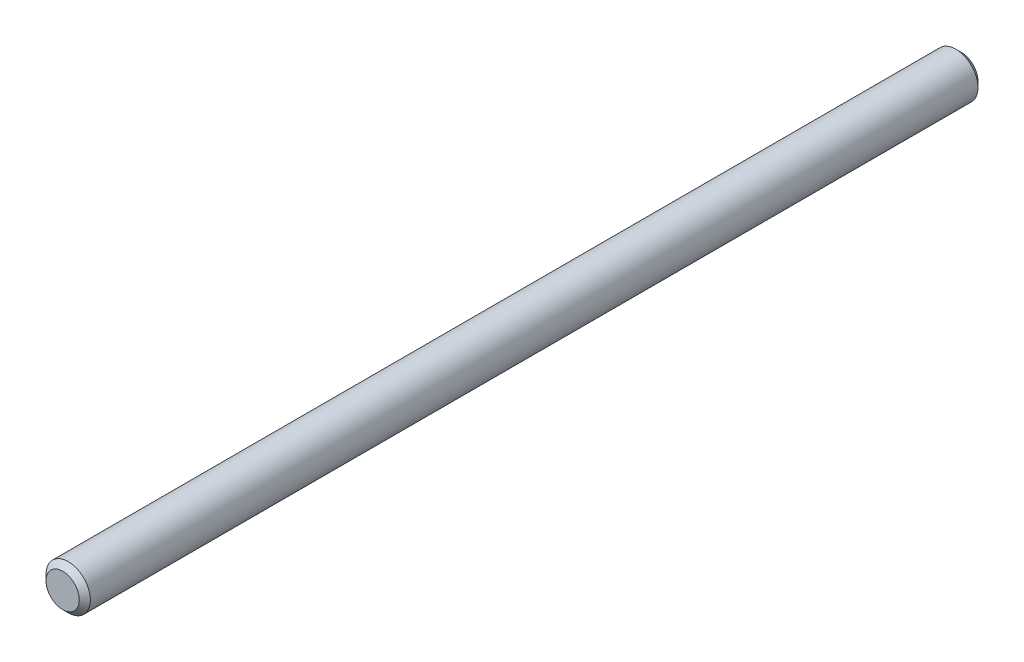
SolidWorks part; units mm, degrees
ref_plane "Front Plane" through (0, 0, 0) normal (0, 0, 1) x (1, 0, 0)
ref_plane "Top Plane" through (0, 0, 0) normal (0, 1, 0) x (1, 0, 0)
ref_plane "Right Plane" through (0, 0, 0) normal (1, 0, 0) x (0, 0, -1)
sketch "Sketch1" plane through (0, 0, 0) normal (0, 0, 1) x (1, 0, 0)
  circle A0 centre (0, 0) radius 0.4
  dimension "D1" = 0.8
extrude "Boss-Extrude1" add sketch "Sketch1" along normal blind 16.2
chamfer "Chamfer1" distance 0.1 angle 45 2 edges at (0.4, 0, 16.2) (0.4, 0, 0)
